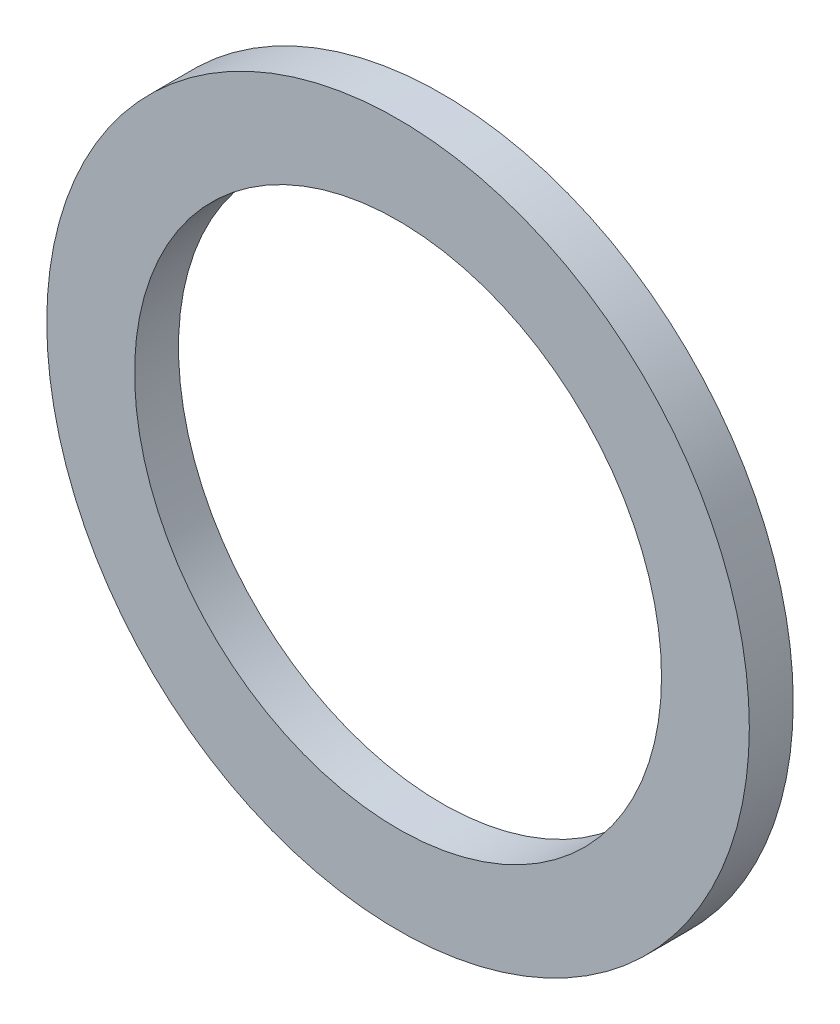
from build123d import *

# Parameters (mm, degrees)
SKETCH_1_R      = 4
SKETCH_1_R_2    = 3
EXTRUDE_1_DEPTH = 0.5


with BuildPart() as part:
    # 草图1 → 凸台-拉伸1 (new body)
    with BuildSketch(Plane.XY):
        Circle(SKETCH_1_R)
        Circle(SKETCH_1_R_2, mode=Mode.SUBTRACT)
    extrude(amount=EXTRUDE_1_DEPTH)


solid = part.part
